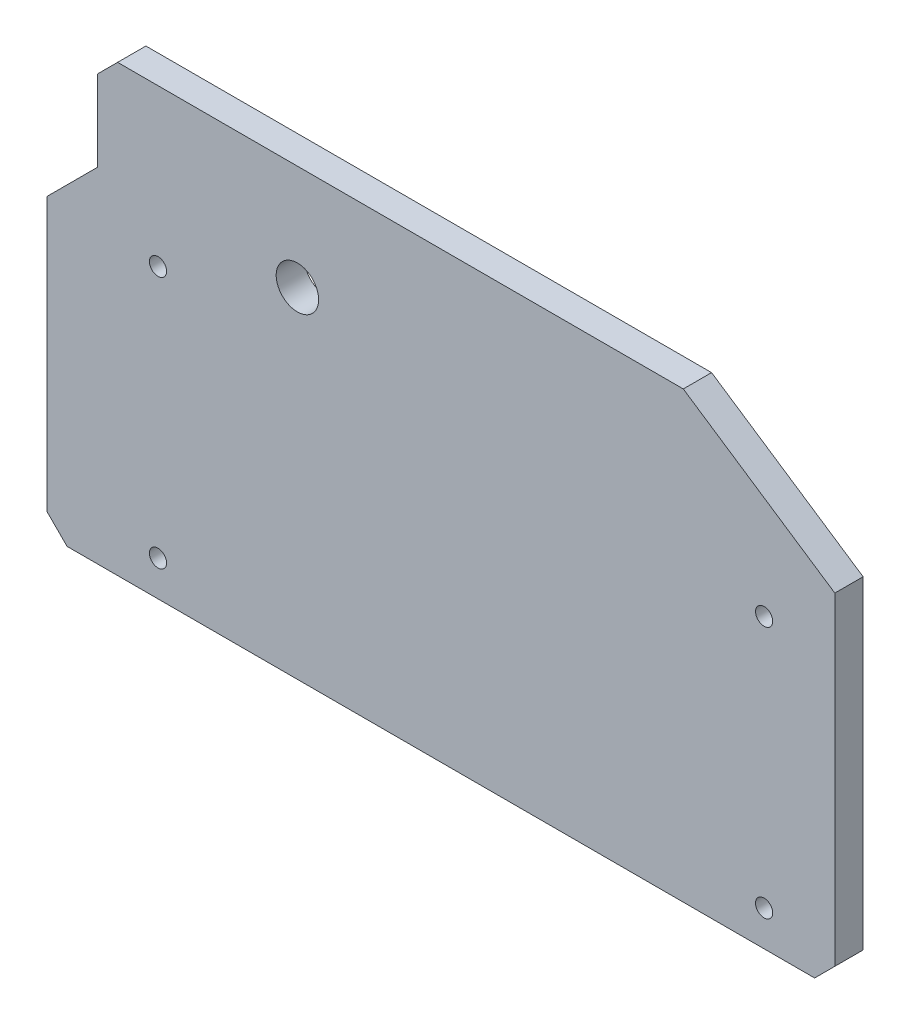
from build123d import *

# Parameters (mm, degrees)
SKETCH1_R           = 10.5
BOSS_EXTRUDE1_DEPTH = 14
M10_TAPPED_HOLE1_D  = 8.5
SKETCH4_W           = 25
SKETCH4_H           = 60
CUT_EXTRUDE1_DEPTH  = 448.99107134
CHAMFER1_SIZE       = 10
CUT_EXTRUDE2_DEPTH  = 448.99107134


with BuildPart() as part:
    # Sketch1 → Boss-Extrude1 (new body)
    with BuildSketch(Plane.XY):
        Polygon((0, 220), (315, 220), (390, 170), (390, 0), (0, 0), align=None)
        with Locations((124, 168)):
            Circle(SKETCH1_R, mode=Mode.SUBTRACT)
    extrude(amount=BOSS_EXTRUDE1_DEPTH)

    # M10 Tapped Hole1 (through all)
    with Locations(Plane.XY.offset(14)):
        with Locations((55, 142.5), (55, 17.5), (355, 142.5), (355, 17.5)):
            Hole(M10_TAPPED_HOLE1_D / 2)

    # Sketch4 → Cut-Extrude1 (cut, through all)
    with BuildSketch(Plane.XY.offset(14)):
        with Locations((12.5, 190)):
            Rectangle(SKETCH4_W, SKETCH4_H)
    extrude(amount=-CUT_EXTRUDE1_DEPTH, mode=Mode.SUBTRACT)

    # Chamfer1
    chamfer1_edges = [part.edges().sort_by_distance(p)[0] for p in [
        (25, 220, 7),
        (25, 160, 7),
        (390, 0, 7),
        (0, 0, 7),
    ]]
    chamfer(chamfer1_edges, length=CHAMFER1_SIZE)

    # Sketch5 → Cut-Extrude2 (cut, through all)
    with BuildSketch(Plane.XY.offset(14)):
        Polygon((15, 160), (0, 160), (0, 145), align=None)
    extrude(amount=-CUT_EXTRUDE2_DEPTH, mode=Mode.SUBTRACT)


solid = part.part
